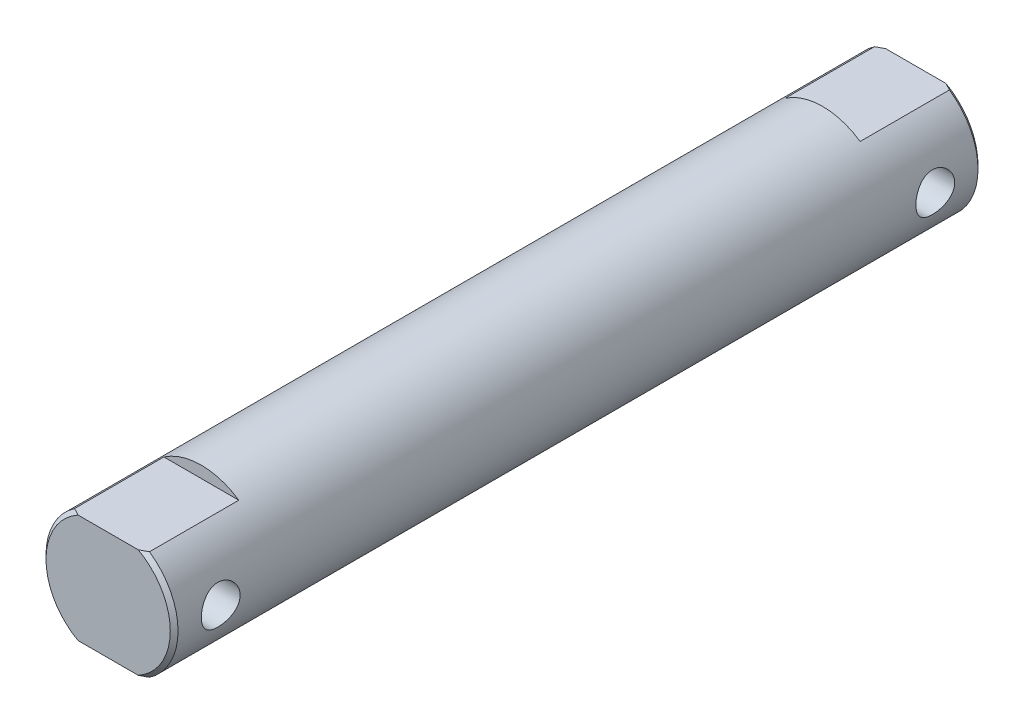
from build123d import *

# Parameters (mm, degrees)
SKETCH_1_R          = 8.5
EXTRUDE_1_DEPTH     = 52
SKETCH_2_W          = 25
SKETCH_2_H          = 3
CUT_EXTRUDE_1_DEPTH = 12
CHAMFER_2_SIZE      = 0.5
HOLE_WIZARD_M6_1_D  = 5


with BuildPart() as part:
    # 草图1 → 凸台-拉伸1 (new, symmetric)
    with BuildSketch(Plane.XY):
        with Locations(Location((0, 0, 0), (0, 0, 180))):
            Circle(SKETCH_1_R)
    extrude(amount=EXTRUDE_1_DEPTH, both=True)

    # 草图2 → 切除-拉伸1 (cut)
    with BuildSketch(Plane.XY.offset(52)):
        with Locations((0, 8.5)):
            Rectangle(SKETCH_2_W, SKETCH_2_H)
        with Locations((0, -8.5)):
            Rectangle(SKETCH_2_W, SKETCH_2_H)
    cut_extrude_1 = extrude(amount=-CUT_EXTRUDE_1_DEPTH, mode=Mode.SUBTRACT)

    # 镜向1: 切除-拉伸1 across plane
    add(cut_extrude_1.mirror(Plane.XY), mode=Mode.SUBTRACT)

    # 倒角2
    chamfer_2_edges = [part.edges().sort_by_distance(p)[0] for p in [
        (8.5, 0, 52),
        (-7.524477249, 3.953763034, -52),
        (8.5, 0, -52),
        (-7.524477249, 3.953763034, 52),
    ]]
    chamfer(chamfer_2_edges, length=CHAMFER_2_SIZE)

    # M6 螺纹孔1 (through all)
    with Locations(Plane(origin=(8.5, 0, 0), x_dir=(0, 0, -1), z_dir=(1, 0, 0))):
        with Locations((-46, 0), (46, 0)):
            Hole(HOLE_WIZARD_M6_1_D / 2)


solid = part.part
